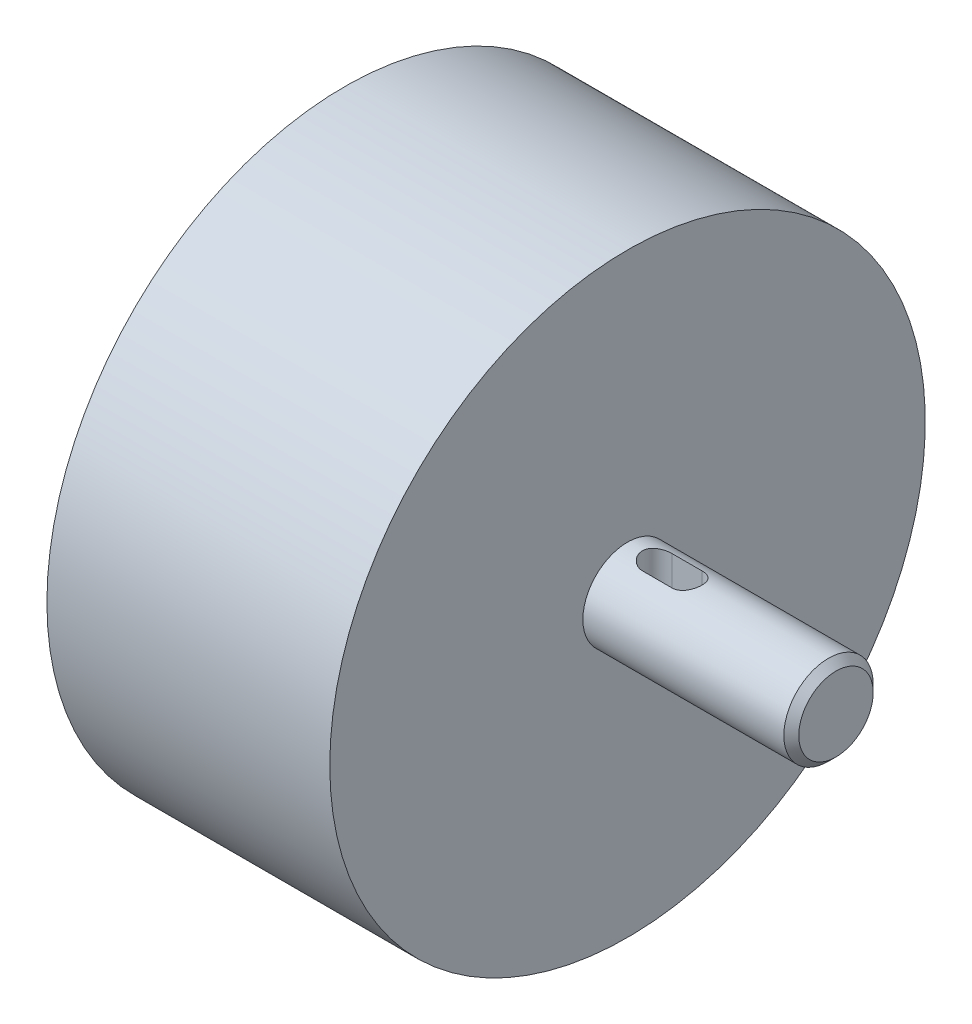
from build123d import *

# Parameters (mm, degrees)
SKETCH2_W               = 13.5
SKETCH2_H               = 13.5
CUT_EXTRUDE1_DEPTH      = 9
CHAMFER1_SIZE           = 1
CUT_EXTRUDE2_DEPTH      = 35.073450075
CUT_EXTRUDE2_DEPTH_BACK = 35.073450075
CHAMFER2_SIZE           = 0.5


with BuildPart() as part:
    # Sketch1 → Revolve1 (revolve)
    with BuildSketch(Plane(origin=(0, 0, 0), x_dir=(1, 0, 0), z_dir=(0, 1, 0))):
        Polygon((0, -3), (14, -3), (14, 0), (-19, 0), (-19, -20), (0, -20), align=None)
    revolve(axis=Axis((-19, 0, 0), (1, 0, 0)))

    # Sketch2 → Cut-Extrude1 (cut)
    with BuildSketch(Plane(origin=(-19, 0, 0), x_dir=(0, 0, -1), z_dir=(1, 0, 0))):
        Rectangle(SKETCH2_W, SKETCH2_H)
    extrude(amount=CUT_EXTRUDE1_DEPTH, mode=Mode.SUBTRACT)

    # Chamfer1
    chamfer1_edges = [part.edges().sort_by_distance(p)[0] for p in [
        (-19, 0, 6.75),
        (-19, -6.75, 0),
        (-19, 0, -6.75),
        (-19, 6.75, 0),
    ]]
    chamfer(chamfer1_edges, length=CHAMFER1_SIZE)

    # Sketch3 → Cut-Extrude2 (cut, two sides: drawn at the far end of the back side and taken through both)
    with BuildSketch(Plane(origin=(0, 0, 0), x_dir=(1, 0, 0), z_dir=(0, 1, 0)).offset(-CUT_EXTRUDE2_DEPTH_BACK)):
        with BuildLine():
            Line((2, 1), (4, 1))
            ThreePointArc((4, 1), (5, 0), (4, -1))
            Line((4, -1), (2, -1))
            ThreePointArc((2, -1), (1, 0), (2, 1))
        make_face()
    extrude(amount=CUT_EXTRUDE2_DEPTH + CUT_EXTRUDE2_DEPTH_BACK, mode=Mode.SUBTRACT)

    # Chamfer2
    chamfer2_edges = [part.edges().sort_by_distance(p)[0] for p in [
        (14, 0, -3),
    ]]
    chamfer(chamfer2_edges, length=CHAMFER2_SIZE)


solid = part.part
